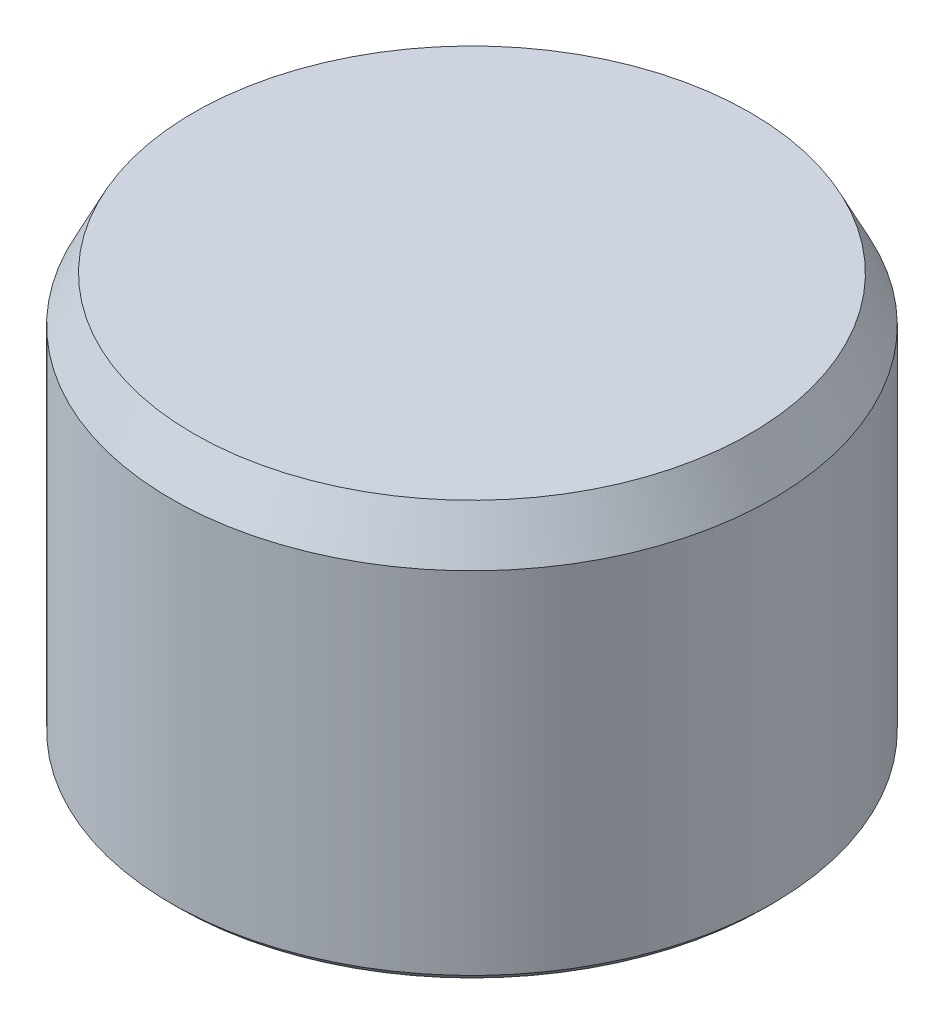
SolidWorks part; units mm, degrees
material "AISI 1045 钢，冷拔"
ref_plane "Front Plane" through (0, 0, 0) normal (0, 0, 1) x (1, 0, 0)
ref_plane "Top Plane" through (0, 0, 0) normal (0, 1, 0) x (1, 0, 0)
ref_plane "Right Plane" through (0, 0, 0) normal (1, 0, 0) x (0, 0, -1)
sketch "Sketch1" plane through (0, 0, 0) normal (0, 0, 1) x (1, 0, 0)
  line L0 (58.9461, 0) -> (0, 0) construction
  line L1 (0, 0) -> (0, 89.3907) construction
  line L3 (20, -13.4) -> (0, -13.4)
  line L4 (20, -13.4) -> (20, 13.4)
  line L5 (20, 13.4) -> (0, 13.4)
  line L6 (0, -13.4) -> (0, 13.4)
  line L7 (20, -13.4) -> (0, 13.4) construction
  line L8 (20, 13.4) -> (0, -13.4) construction
  point P3 (10, 0)
  dimension "D1" = 26.8
  dimension "D2" = 40
revolve "Revolve1" add sketch "Sketch1" angle 360 about L1
chamfer "Chamfer1" distance 1.5 distance2 3 1 edges at (0, 13.4, -20)
chamfer "Chamfer2" distance 0.5 angle 45 1 edges at (0, -13.4, -20)
